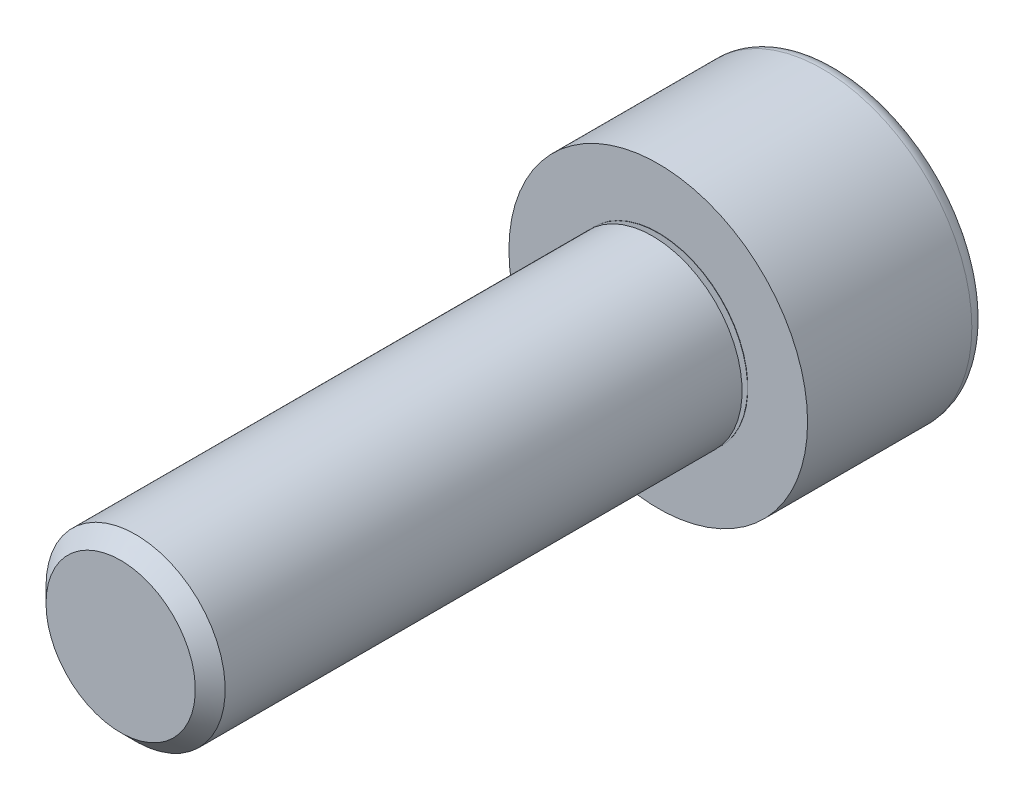
from build123d import *

# Parameters (mm, degrees)
CUT_EXTRUDE1_DEPTH = 2.5


with BuildPart() as part:
    # Logo3_bib1 → Revolve1 (revolve)
    with BuildSketch(Plane(origin=(0, 0, 0), x_dir=(-1, 0, 0), z_dir=(0, -1, 0))):
        with BuildLine():
            Line((0, -18), (0, 6))
            Line((0, 6), (4.5, 6))
            ThreePointArc((4.5, 6), (4.853553391, 5.853553391), (5, 5.5))
            Line((5, 5.5), (5, 0))
            Line((5, 0), (3, 0))
            Line((3, 0), (3, -0.01))
            Line((3, -0.01), (2.613425636, -0.01))
            ThreePointArc((2.613425636, -0.01), (2.593729481, -0.026527036), (2.606585234, -0.048793852))
            Line((2.606585234, -0.048793852), (3, -0.191985117))
            Line((3, -0.191985117), (3, -17.5))
            Line((3, -17.5), (2.5, -18))
            Line((2.5, -18), (0, -18))
        make_face()
    revolve(axis=Axis((0, 0, -10.585154653), (0, 0, 1)))

    # Logo3_bib2 → Cut-Extrude1 (cut)
    with BuildSketch(Plane(origin=(0, 0, -6), x_dir=(1, 0, 0), z_dir=(0, 0, -1))):
        Polygon((2.886751346, 0), (1.443375673, 2.5), (-1.443375673, 2.5), (-2.886751346, 0), (-1.443375673, -2.5), (1.443375673, -2.5), align=None)
    extrude(amount=-CUT_EXTRUDE1_DEPTH, mode=Mode.SUBTRACT)


solid = part.part
